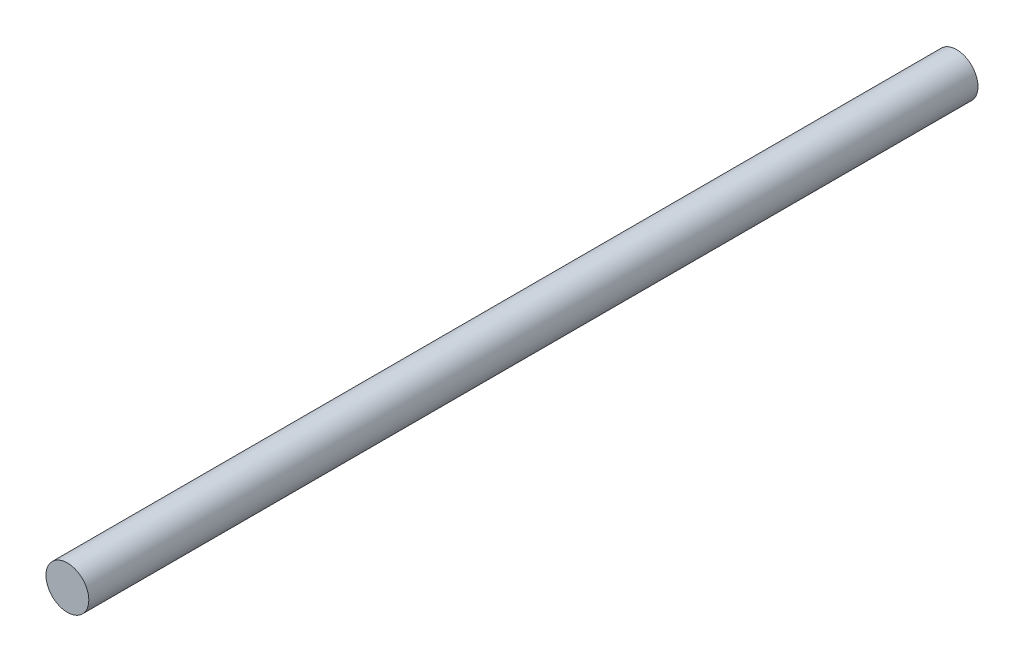
SolidWorks part; units mm, degrees
material "Stainless Steel (ferritic)"
ref_plane "Front Plane" through (0, 0, 0) normal (0, 0, 1) x (1, 0, 0)
ref_plane "Top Plane" through (0, 0, 0) normal (0, 1, 0) x (1, 0, 0)
ref_plane "Right Plane" through (0, 0, 0) normal (1, 0, 0) x (0, 0, -1)
sketch "Sketch1" plane through (0, 0, 0) normal (0, 0, 1) x (1, 0, 0)
  circle A0 centre (0, 0) radius 6
  dimension "D1" = 12
extrude "Boss-Extrude1" add sketch "Sketch1" along normal mid plane 249
